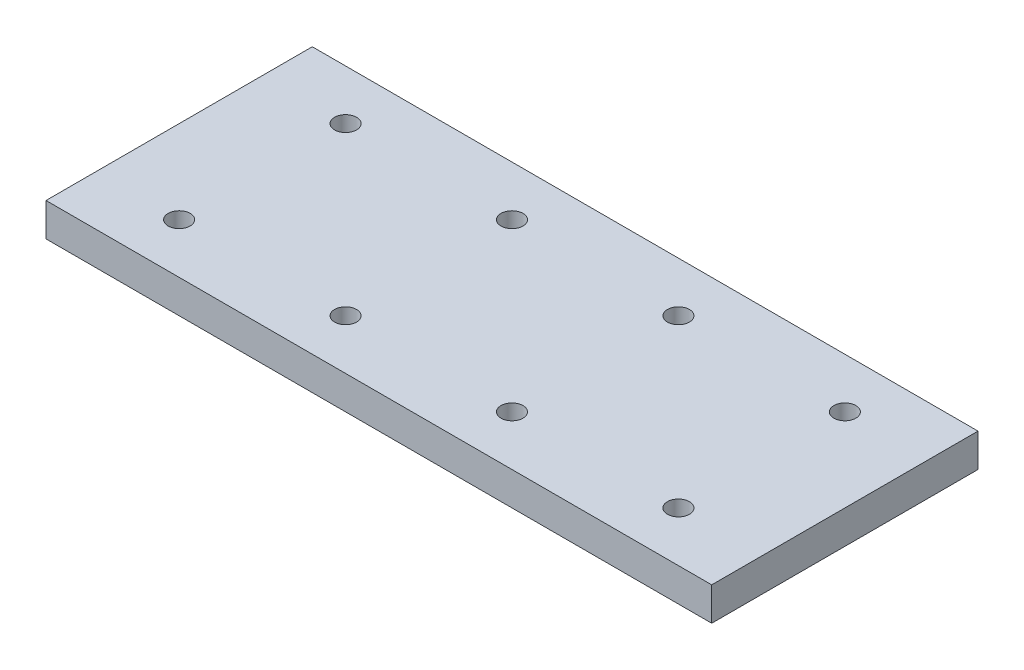
from build123d import *

# Parameters (mm, degrees)
SKETCH1_W                  = 200
SKETCH1_H                  = 80
BOSS_EXTRUDE1_DEPTH        = 10
F_6_6_6_6_DIAMETER_HOLE1_D = 6.6


with BuildPart() as part:
    # Sketch1 → Boss-Extrude1 (new body)
    with BuildSketch(Plane(origin=(0, 0, 0), x_dir=(1, 0, 0), z_dir=(0, 1, 0))):
        Rectangle(SKETCH1_W, SKETCH1_H)
    extrude(amount=BOSS_EXTRUDE1_DEPTH)

    # Ø6.6 (6.6) Diameter Hole1 (through all)
    with Locations(Plane(origin=(0, 10, 0), x_dir=(1, 0, 0), z_dir=(0, 1, 0))):
        with Locations((-25, 25), (25, 25), (-25, -25), (25, -25), (-75, 25), (75, 25), (75, -25), (-75, -25)):
            Hole(F_6_6_6_6_DIAMETER_HOLE1_D / 2)


solid = part.part
